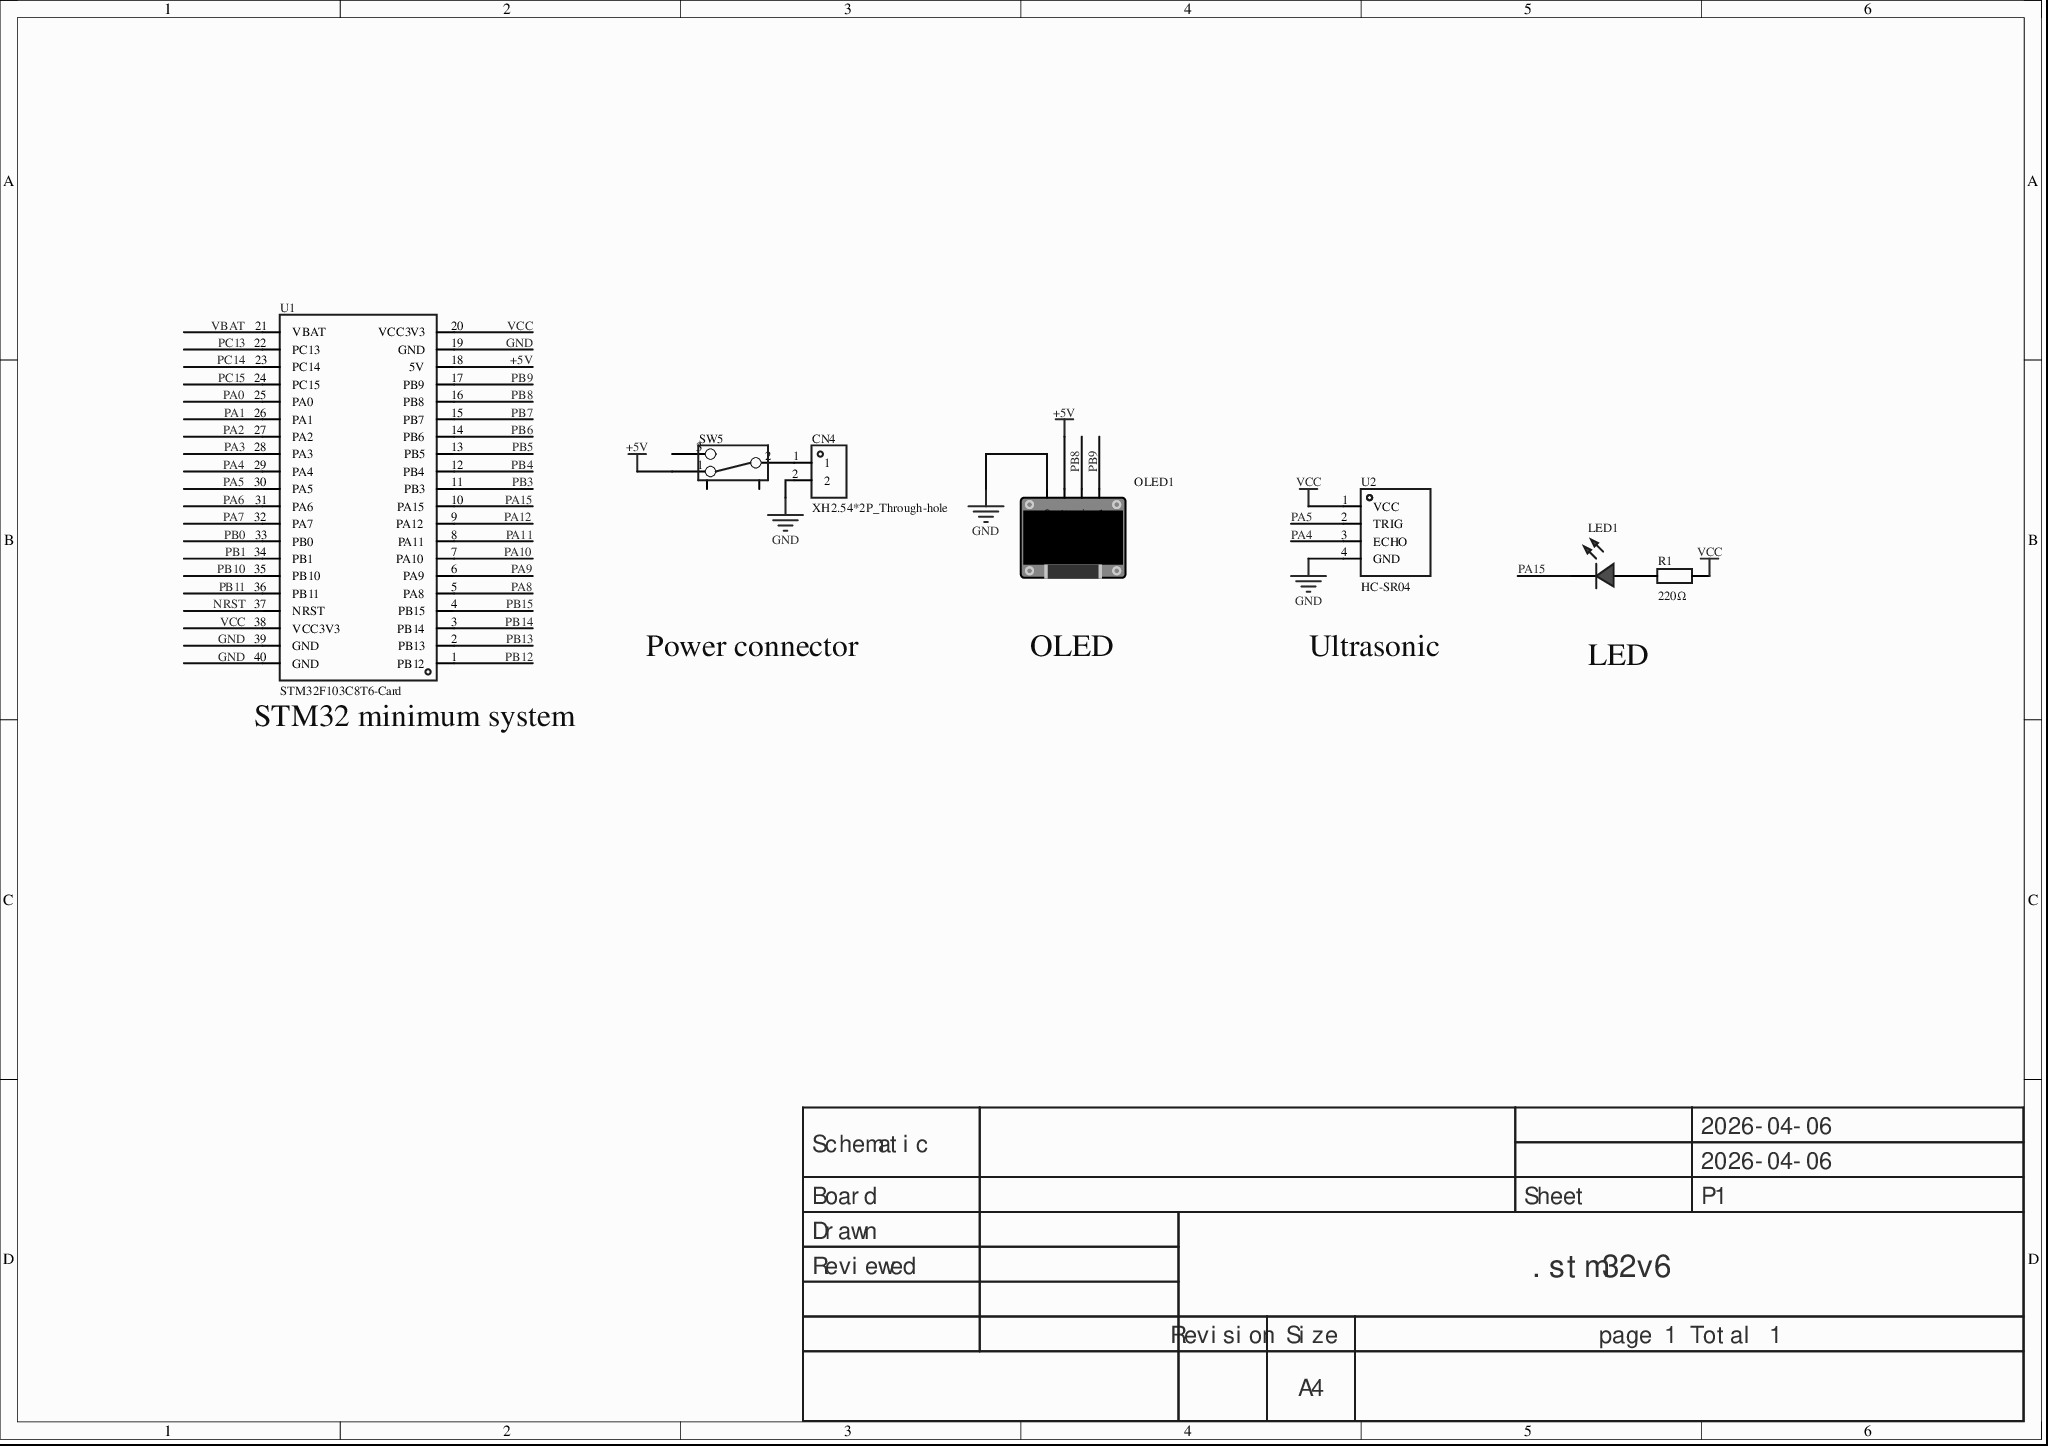
[diagram p0: MISC89090-3.schdoc]
# Altium project MISC89090-2.PrjPcb
1 sheet, 7 parts. Net scope: global (net labels, ports and power ports of the same name join across sheets).
Board file: MISC89090.pcbdoc

## Sheet MISC89090-3.schdoc
size 297 x 209 mm; Version: V1.0; @Project Name: MISC89090; @Page Count: 1; @Update Date: 2026-04-06; @Create Date: 2026-04-06; @Schematic Name: MISC89090; @Page No: 1; @Create Time: 23:22:16; @Update Time: 17:32:40; @Board Name: MISC89090

### Parts
CN4  XH2.54*2P_Through-hole  [CONN-TH_2P-P2.50-XH2.54-2P]
LED1  (no value)  [LED_TH-3mm]
OLED1  (no value)  [0.96OLED_4P]
R1  220Ω  [Res_1/8W]
SW5  (no value)  [拨动开关]
U1  STM32F103C8T6-Card  [CONN-TH_L53.3-W22.9_STM32F103C8T6-CARD]
U2  HC-SR04  [TH_HC-SR04V]

### Nets
+5V: OLED1.2(VCC) SW5.1 U1.18(5V)
GND: CN4.2 OLED1.1(GND) U1.19(GND) U1.39(GND) U1.40(GND) U2.4(GND)
VCC: R1.2 U1.20(VCC3V3) U1.38(VCC3V3) U2.1(VCC)
NRST: U1.37(NRST)
PA0: U1.25(PA0)
PA1: U1.26(PA1)
PA2: U1.27(PA2)
PA3: U1.28(PA3)
PA4: U1.29(PA4) U2.3(ECHO)
PA5: U1.30(PA5) U2.2(TRIG)
PA6: U1.31(PA6)
PA7: U1.32(PA7)
PA8: U1.5(PA8)
PA9: U1.6(PA9)
PA10: U1.7(PA10)
PA11: U1.8(PA11)
PA12: U1.9(PA12)
PA15: LED1.2(A) U1.10(PA15)
PB0: U1.33(PB0)
PB1: U1.34(PB1)
PB3: U1.11(PB3)
PB4: U1.12(PB4)
PB5: U1.13(PB5)
PB6: U1.14(PB6)
PB7: U1.15(PB7)
PB8: OLED1.3(SCL) U1.16(PB8)
PB9: OLED1.4(SDA) U1.17(PB9)
PB10: U1.35(PB10)
PB11: U1.36(PB11)
PB12: U1.1(PB12)
PB13: U1.2(PB13)
PB14: U1.3(PB14)
PB15: U1.4(PB15)
PC13: U1.22(PC13)
PC14: U1.23(PC14)
PC15: U1.24(PC15)
VBAT: U1.21(VBAT)
NetCN4_1: CN4.1 SW5.2
NetLED1_1: LED1.1(C) R1.1

Not connected (* = marked no-connect by the designer): SW5 3 4 5

### Notes on the sheet
- Power connector
- OLED
- Ultrasonic
- LED
- (near U1) STM32 minimum system
- 2026-04-06
- Schematic
- Board
- Sheet
- P1
- Drawn
- Reviewed
- .stm32v6
- Revision
- Size
- A4
- page 1 Total 1

### Library data of the parts
CN4 = XH2.54*2P_直插: 3D Model: 325c595e30db4df8abe76612dd40b0fa0819f05c4eef4c71ace90d822a990e87; 3D Model Transform: 295.275,228.346,0,180,0,0,-0.002,-20.079,-137.795; AddInBom: yes; Symbol: XH2.54*2P_Through-hole; Device: XH2.54*2P_Through-hole; LCSC Part Name: XH2.54*2P_直插; Supplier Part: C9900008615; Manufacturer Part: XH2.54*2P_直插; Supplier Footprint: XH2.54_2P; JLCPCB Part Class: Extended Part; Supplier: LCSC; ConvertToPcb: yes; FootprintName: CONN-TH_2P-P2.50-XH2.54-2P; ModelName: CONN-TH_2P-P2.50-XH2.54-2P
LED1 = LED_TH-R_3mm: ConvertToPcb: yes; ModelId: a497c992633541038a38947cdc58012f0819f05c4eef4c71ace90d822a990e87; ModelName: LED-TH-3mm_R; ModelTransform: 141.274,153.327,0,0,0,0,-5.984,0,-137.795; Symbol: LED_TH-R; Device: LED_TH-R_3mm; AddInBom: yes; FootprintName: LED_TH-3mm; Supplier Footprint: 插件
OLED1 = 0.96OLED模块_4P: Symbol: 0.96OLED module_4P; ConvertToPcb: yes; ModelId: 79c000fdb68d45a296c2e9bedf4f9055; ModelTransform: 1393.69792,1318.895,0,0,0,0,0,-560.079,-137.795; Device: 0.96OLED module_4P; AddInBom: yes; FootprintName: 0.96OLED_4P; Supplier Footprint: 插件; ModelName: 0.96OLED_4P
R1 = Res_AXIAL-1/8W: Symbol: Resistor; ConvertToPcb: yes; ModelId: b2b5ae7ae4c642178fe0039925c86a3f0819f05c4eef4c71ace90d822a990e87; ModelName: RES-TH_BD1.8-L3.2-P7.20-D0.4; ModelTransform: 282.86,66.88,253.09,0,0,0,0,0,-191; Device: Res_AXIAL-1/8W; Value: 220Ω; AddInBom: yes; Supplier Footprint: 轴向引线; FootprintName: Res_1/8W
SW5 = 拨动开关_正: Symbol: Toggle switch; Device: Toggle switch_positive; ConvertToPcb: yes; ModelId: 4321fe59a4074cbfb4989553f297c68f0819f05c4eef4c71ace90d822a990e87; ModelName: SW-TH_SS-12D02-VG4; ModelTransform: 370.09,208.7,472.35,0,0,0,0,0,-110; AddInBom: yes; Supplier Footprint: 插件; FootprintName: Toggle switch
U1 = STM32F103C8T6-Card: AddInBom: yes; Symbol: STM32F103C8T6-CARD; Device: STM32F103C8T6-Card; LCSC Part Name: STM32F103C8T6-Card; SupplierPart: C9900077949; ManufacturerPart: STM32F103C8T6-Card; Supplier Footprint: 插件; Supplier: LCSC; ConvertToPcb: yes; FootprintName: CONN-TH_L53.3-W22.9_STM32F103C8T6-CARD
U2 = HC-SR04: Manufacturer: Universal Microelectronics; AddInBom: yes; Symbol: HC-SR04; Device: HC-SR04; LCSC Part Name: HC-SR04; SupplierPart: C19857336; ManufacturerPart: HC-SR04; Supplier Footprint: -; JLCPCB Part Class: Extended library; Datasheet: https://atta.szlcsc.com/upload/public/pdf/source/20240122/47B8E374E428935B7962A2189EF91AAC.pdf; Supplier: LCSC; ConvertToPcb: yes; FootprintName: TH_HC-SR04V